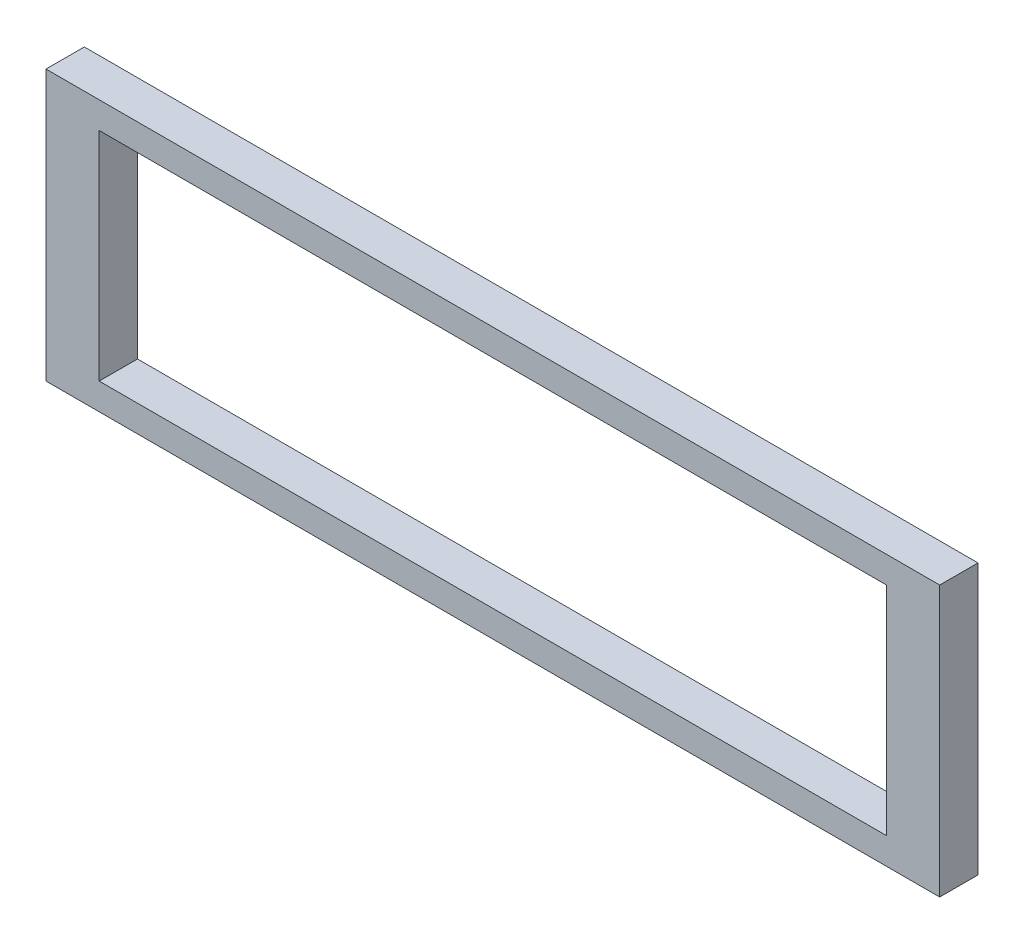
from build123d import *

# Parameters (mm, degrees)
SKETCH_1_W      = 420
SKETCH_1_H      = 127
SKETCH_1_W_2    = 370
SKETCH_1_H_2    = 102
EXTRUDE_1_DEPTH = 9


with BuildPart() as part:
    # 草图1 → 凸台-拉伸1 (new, symmetric)
    with BuildSketch(Plane.XY):
        Rectangle(SKETCH_1_W, SKETCH_1_H)
        Rectangle(SKETCH_1_W_2, SKETCH_1_H_2, mode=Mode.SUBTRACT)
    extrude(amount=EXTRUDE_1_DEPTH, both=True)


solid = part.part
